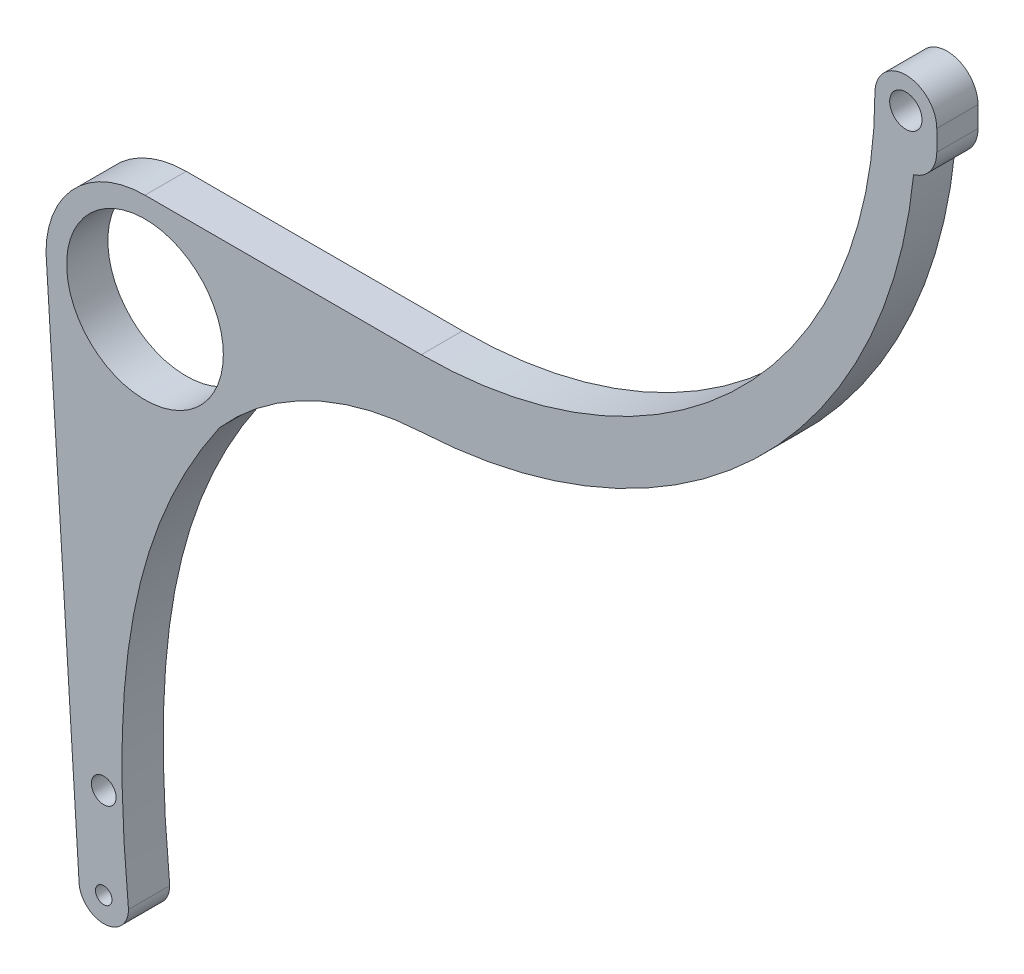
from build123d import *

# Parameters (mm, degrees)
SKETCH_1_R      = 2
SKETCH_1_R_2    = 19
SKETCH_1_R_3    = 3.91899873
SKETCH_1_R_4    = 3
EXTRUDE_3_DEPTH = 10


with BuildPart() as part:
    # 草图1 → 凸台-拉伸3 (new body)
    with BuildSketch(Plane.XY):
        with BuildLine():
            Line((-14, 128), (-6, 0))
            ThreePointArc((-6, 0), (0, -6), (6, 0))
            add(Edge.make_bspline(
                [(6, 0), (1.588652615, 45.680929706), (5.604102499, 79.643200211), (28.004797731, 112.13093391)],
                knots=[0, 0, 0, 0, 0.788155359, 0.788155359, 0.788155359, 0.788155359], degree=3))
            ThreePointArc((28.004797731, 112.13093391), (50.113637924, 128.900750568), (77, 135.767416406))
            ThreePointArc((77, 135.767416406), (157.787149523, 170.485384951), (196.379869136, 249.494896157))
            ThreePointArc((196.379869136, 249.494896157), (200.439238403, 252.311917913), (202, 257))
            Line((202, 257), (202, 262))
            ThreePointArc((202, 262), (194.5, 269.5), (187, 262))
            ThreePointArc((187, 262), (154.781745931, 184.218254069), (77, 152))
            Line((77, 152), (10, 152))
            ThreePointArc((10, 152), (-6.970562748, 144.970562748), (-14, 128))
        make_face()
        Circle(SKETCH_1_R, mode=Mode.SUBTRACT)
        with Locations((10, 128)):
            Circle(SKETCH_1_R_2, mode=Mode.SUBTRACT)
        with Locations((194.5, 262)):
            Circle(SKETCH_1_R_3, mode=Mode.SUBTRACT)
        with Locations((0, 22)):
            Circle(SKETCH_1_R_4, mode=Mode.SUBTRACT)
    extrude(amount=EXTRUDE_3_DEPTH)


solid = part.part
